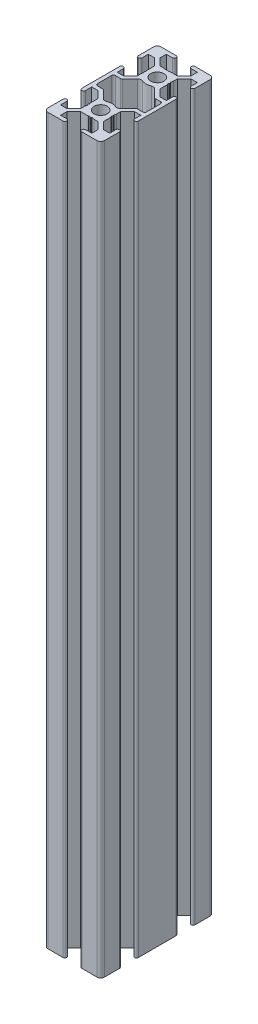
from build123d import *

# Parameters (mm, degrees)
SKETCH11_R                             = 3.4
ALUMINIUM_PROFILE_30_X_60_X_R2_1_DEPTH = 384
M8X1_0_TAPPED_HOLE1_D                  = 7
M8X1_0_TAPPED_HOLE1_DEPTH              = 389
M8X1_0_TAPPED_HOLE1_TIP                = 2.103012167
M8X1_0_TAPPED_HOLE2_D                  = 7
M8X1_0_TAPPED_HOLE2_DEPTH              = 15
M8X1_0_TAPPED_HOLE2_TIP                = 2.103012167


with BuildPart() as part:
    # Sketch11 → Aluminium profile 30 X 60 X R2(1) (new body)
    with BuildSketch(Plane(origin=(0, 0, 0), x_dir=(1, 0, 0), z_dir=(0, 1, 0))):
        with BuildLine():
            Line((-15, -20), (-15, -28))
            ThreePointArc((-15, -28), (-14.414213562, -29.414213562), (-13, -30))
            Line((-13, -30), (-5, -30))
            ThreePointArc((-5, -30), (-4, -29), (-5, -28))
            Line((-5, -28), (-8.25, -28))
            Line((-8.25, -28), (-8.25, -24.664213562))
            Line((-8.25, -24.664213562), (-4.585786438, -21))
            Line((-4.585786438, -21), (-0.653589838, -21))
            ThreePointArc((-0.653589838, -21), (-0.524180316, -20.982962913), (-0.403589838, -20.933012702))
            Line((-0.403589838, -20.933012702), (0, -20.7))
            Line((0, -20.7), (0.403589838, -20.933012702))
            ThreePointArc((0.403589838, -20.933012702), (0.653589838, -21), (0.903589838, -20.933012702))
            Line((0.903589838, -20.933012702), (1.218885629, -20.750976592))
            Line((1.218885629, -20.750976592), (2.5, -21))
            Line((2.5, -21), (4.585786438, -21))
            Line((4.585786438, -21), (8.25, -24.664213562))
            Line((8.25, -24.664213562), (8.25, -28))
            Line((8.25, -28), (5, -28))
            ThreePointArc((5, -28), (4, -29), (5, -30))
            Line((5, -30), (13, -30))
            ThreePointArc((13, -30), (14.414213562, -29.414213562), (15, -28))
            Line((15, -28), (15, -20.00000006))
            ThreePointArc((15, -20.00000006), (14, -19.00000006), (13, -20.00000006))
            Line((13, -20.00000006), (13, -23.25))
            Line((13, -23.25), (9.664213562, -23.25))
            Line((9.664213562, -23.25), (6, -19.585786438))
            Line((6, -19.585786438), (6, -15.653589838))
            ThreePointArc((6, -15.653589838), (5.982962913, -15.524180316), (5.933012702, -15.403589838))
            Line((5.933012702, -15.403589838), (5.7, -15))
            Line((5.7, -15), (5.933012702, -14.596410162))
            ThreePointArc((5.933012702, -14.596410162), (6, -14.346410162), (5.933012702, -14.096410162))
            Line((5.933012702, -14.096410162), (5.750976592, -13.781114371))
            Line((5.750976592, -13.781114371), (6, -12.5))
            Line((6, -12.5), (6, -10.414213562))
            Line((6, -10.414213562), (9.664213562, -6.75))
            Line((9.664213562, -6.75), (13, -6.75))
            Line((13, -6.75), (13, -9.999999769))
            ThreePointArc((13, -9.999999769), (14, -10.999999769), (15, -9.999999769))
            Line((15, -9.999999769), (15, 9.99999994))
            ThreePointArc((15, 9.99999994), (14, 10.99999994), (13, 9.99999994))
            Line((13, 9.99999994), (13, 6.75))
            Line((13, 6.75), (9.664213562, 6.75))
            Line((9.664213562, 6.75), (6, 10.414213562))
            Line((6, 10.414213562), (6, 14.346410162))
            ThreePointArc((6, 14.346410162), (5.982962913, 14.475819684), (5.933012702, 14.596410162))
            Line((5.933012702, 14.596410162), (5.7, 15))
            Line((5.7, 15), (5.933012702, 15.403589838))
            ThreePointArc((5.933012702, 15.403589838), (6, 15.653589838), (5.933012702, 15.903589838))
            Line((5.933012702, 15.903589838), (5.750976592, 16.218885629))
            Line((5.750976592, 16.218885629), (6, 17.5))
            Line((6, 17.5), (6, 19.585786438))
            Line((6, 19.585786438), (9.664213562, 23.25))
            Line((9.664213562, 23.25), (13, 23.25))
            Line((13, 23.25), (13, 20))
            ThreePointArc((13, 20), (14, 19), (15, 20))
            Line((15, 20), (15, 28))
            ThreePointArc((15, 28), (14.414213562, 29.414213562), (13, 30))
            Line((13, 30), (5, 30))
            ThreePointArc((5, 30), (4, 29), (5, 28))
            Line((5, 28), (8.25, 28))
            Line((8.25, 28), (8.25, 24.664213562))
            Line((8.25, 24.664213562), (4.585786438, 21))
            Line((4.585786438, 21), (0.653589838, 21))
            ThreePointArc((0.653589838, 21), (0.524180316, 20.982962913), (0.403589838, 20.933012702))
            Line((0.403589838, 20.933012702), (0, 20.7))
            Line((0, 20.7), (-0.403589838, 20.933012702))
            ThreePointArc((-0.403589838, 20.933012702), (-0.653589838, 21), (-0.903589838, 20.933012702))
            Line((-0.903589838, 20.933012702), (-1.218885629, 20.750976592))
            Line((-1.218885629, 20.750976592), (-2.5, 21))
            Line((-2.5, 21), (-4.585786438, 21))
            Line((-4.585786438, 21), (-8.25, 24.664213562))
            Line((-8.25, 24.664213562), (-8.25, 28))
            Line((-8.25, 28), (-5, 28))
            ThreePointArc((-5, 28), (-4, 29), (-5, 30))
            Line((-5, 30), (-13, 30))
            ThreePointArc((-13, 30), (-14.414213562, 29.414213562), (-15, 28))
            Line((-15, 28), (-15, 20))
            ThreePointArc((-15, 20), (-14, 19), (-13, 20))
            Line((-13, 20), (-13, 23.25))
            Line((-13, 23.25), (-9.664213562, 23.25))
            Line((-9.664213562, 23.25), (-6, 19.585786438))
            Line((-6, 19.585786438), (-6, 15.653589838))
            ThreePointArc((-6, 15.653589838), (-5.982962913, 15.524180316), (-5.933012702, 15.403589838))
            Line((-5.933012702, 15.403589838), (-5.7, 15))
            Line((-5.7, 15), (-5.933012702, 14.596410162))
            ThreePointArc((-5.933012702, 14.596410162), (-6, 14.346410162), (-5.933012702, 14.096410162))
            Line((-5.933012702, 14.096410162), (-5.750976592, 13.781114371))
            Line((-5.750976592, 13.781114371), (-6, 12.5))
            Line((-6, 12.5), (-6, 10.414213562))
            Line((-6, 10.414213562), (-9.664213562, 6.75))
            Line((-9.664213562, 6.75), (-13, 6.75))
            Line((-13, 6.75), (-13, 9.99999994))
            ThreePointArc((-13, 9.99999994), (-14, 10.99999994), (-15, 9.99999994))
            Line((-15, 9.99999994), (-15, -9.999999769))
            ThreePointArc((-15, -9.999999769), (-14, -10.999999769), (-13, -9.999999769))
            Line((-13, -9.999999769), (-13, -6.75))
            Line((-13, -6.75), (-9.664213562, -6.75))
            Line((-9.664213562, -6.75), (-6, -10.414213562))
            Line((-6, -10.414213562), (-6, -14.346410162))
            ThreePointArc((-6, -14.346410162), (-5.982962913, -14.475819684), (-5.933012702, -14.596410162))
            Line((-5.933012702, -14.596410162), (-5.7, -15))
            Line((-5.7, -15), (-5.933012702, -15.403589838))
            ThreePointArc((-5.933012702, -15.403589838), (-6, -15.653589838), (-5.933012702, -15.903589838))
            Line((-5.933012702, -15.903589838), (-5.750976592, -16.218885629))
            Line((-5.750976592, -16.218885629), (-6, -17.5))
            Line((-6, -17.5), (-6, -19.585786438))
            Line((-6, -19.585786438), (-9.664213562, -23.25))
            Line((-9.664213562, -23.25), (-13, -23.25))
            Line((-13, -23.25), (-13, -20))
            ThreePointArc((-13, -20), (-14, -19), (-15, -20))
        make_face()
        with Locations((0, 15)):
            Circle(SKETCH11_R, mode=Mode.SUBTRACT)
        with Locations((0, -15)):
            Circle(SKETCH11_R, mode=Mode.SUBTRACT)
        with BuildLine():
            Line((-13, 3.75), (-13, -3.75))
            ThreePointArc((-13, -3.75), (-12.707106781, -4.457106781), (-12, -4.75))
            Line((-12, -4.75), (-9.25, -4.75))
            ThreePointArc((-9.25, -4.75), (-8.867316568, -4.826120467), (-8.542893219, -5.042893219))
            Line((-8.542893219, -5.042893219), (-4.53693746, -9.048848978))
            ThreePointArc((-4.53693746, -9.048848978), (-3.504758422, -9.597808771), (-2.342042923, -9.475976562))
            ThreePointArc((-2.342042923, -9.475976562), (0, -9), (2.342042923, -9.475976562))
            ThreePointArc((2.342042923, -9.475976562), (3.504758422, -9.597808771), (4.53693746, -9.048848978))
            Line((4.53693746, -9.048848978), (8.542893219, -5.042893219))
            ThreePointArc((8.542893219, -5.042893219), (8.867316568, -4.826120467), (9.25, -4.75))
            Line((9.25, -4.75), (12, -4.75))
            ThreePointArc((12, -4.75), (12.707106781, -4.457106781), (13, -3.75))
            Line((13, -3.75), (13, 3.75))
            ThreePointArc((13, 3.75), (12.707106781, 4.457106781), (12, 4.75))
            Line((12, 4.75), (9.25, 4.75))
            ThreePointArc((9.25, 4.75), (8.867316568, 4.826120467), (8.542893219, 5.042893219))
            Line((8.542893219, 5.042893219), (4.53693746, 9.048848978))
            ThreePointArc((4.53693746, 9.048848978), (3.504758422, 9.597808771), (2.342042923, 9.475976562))
            ThreePointArc((2.342042923, 9.475976562), (0, 9), (-2.342042923, 9.475976562))
            ThreePointArc((-2.342042923, 9.475976562), (-3.504758422, 9.597808771), (-4.53693746, 9.048848978))
            Line((-4.53693746, 9.048848978), (-8.542893219, 5.042893219))
            ThreePointArc((-8.542893219, 5.042893219), (-8.867316568, 4.826120467), (-9.25, 4.75))
            Line((-9.25, 4.75), (-12, 4.75))
            ThreePointArc((-12, 4.75), (-12.707106781, 4.457106781), (-13, 3.75))
        make_face(mode=Mode.SUBTRACT)
    extrude(amount=ALUMINIUM_PROFILE_30_X_60_X_R2_1_DEPTH)

    # M8x1.0 Tapped Hole1
    with Locations(Plane(origin=(0, 384, 0), x_dir=(1, 0, 0), z_dir=(0, 1, 0))):
        with Locations((0, 15), (0, -15)):
            Hole(M8X1_0_TAPPED_HOLE1_D / 2, depth=M8X1_0_TAPPED_HOLE1_DEPTH)
            with Locations((0, 0, -(M8X1_0_TAPPED_HOLE1_DEPTH + M8X1_0_TAPPED_HOLE1_TIP / 2))):  # 118° drill point
                Cone(0, M8X1_0_TAPPED_HOLE1_D / 2, M8X1_0_TAPPED_HOLE1_TIP, mode=Mode.SUBTRACT)

    # M8x1.0 Tapped Hole2
    with Locations(Plane(origin=(0, 0, -15), x_dir=(0, 0, -1), z_dir=(0, -1, 0))):
        with Locations((0, 0), (-30, 0)):
            Hole(M8X1_0_TAPPED_HOLE2_D / 2, depth=M8X1_0_TAPPED_HOLE2_DEPTH)
            with Locations((0, 0, -(M8X1_0_TAPPED_HOLE2_DEPTH + M8X1_0_TAPPED_HOLE2_TIP / 2))):  # 118° drill point
                Cone(0, M8X1_0_TAPPED_HOLE2_D / 2, M8X1_0_TAPPED_HOLE2_TIP, mode=Mode.SUBTRACT)


solid = part.part
